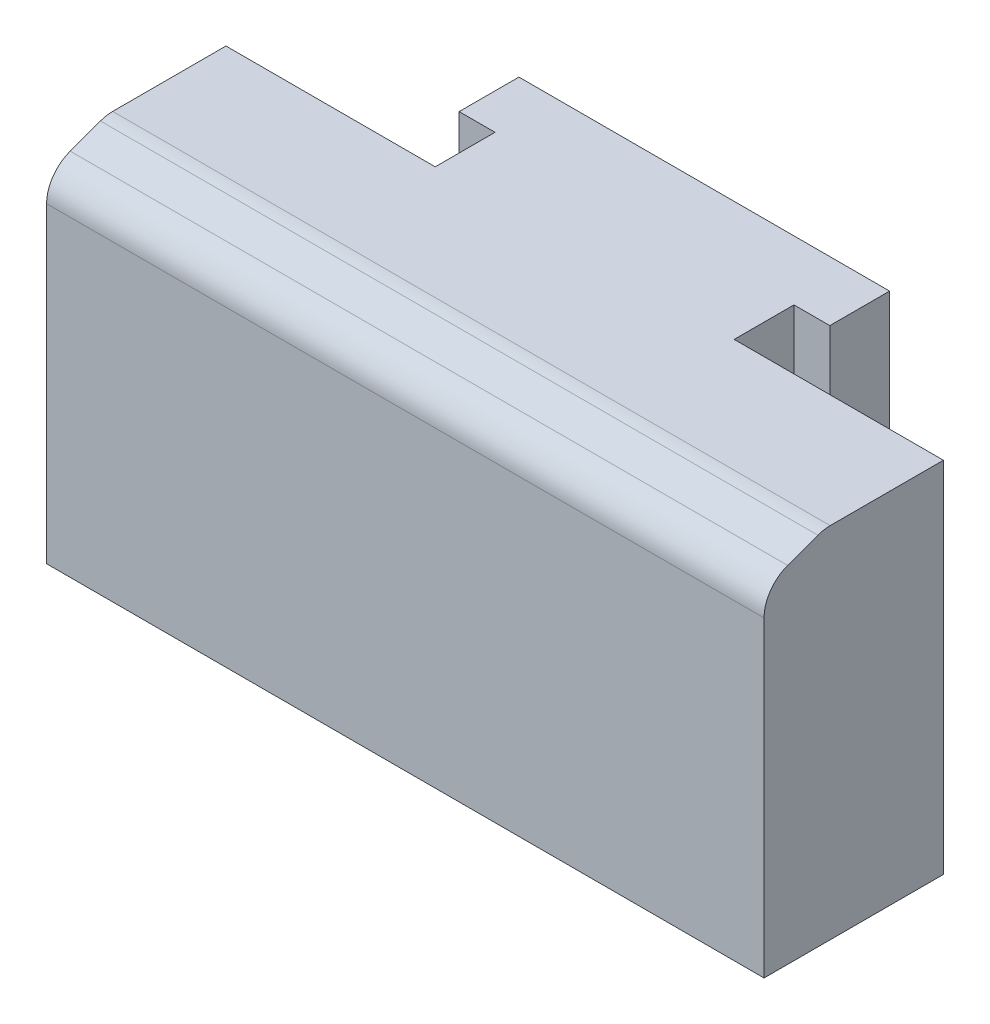
from build123d import *

# Parameters (mm, degrees)
SKETCH1_W              = 31
SKETCH1_H              = 30
BOSS_EXTRUDE1_DEPTH    = 25
SKETCH2_W              = 3
SKETCH2_H              = 20
CUT_EXTRUDE1_DEPTH     = 51.498103381
SKETCH3_W              = 17.5
SKETCH3_H              = 15
BOSS_EXTRUDE2_DEPTH    = 30
CHAMFER1_SIZE          = 5
CHAMFER1_SIZE2         = 1.819851171
FILLET1_R              = 3
M10_TAPPED_HOLE1_D     = 8.5
M10_TAPPED_HOLE1_DEPTH = 24.5
M10_TAPPED_HOLE1_TIP   = 2.553657631


with BuildPart() as part:
    # Sketch1 → Boss-Extrude1 (new body)
    with BuildSketch(Plane.XY):
        with Locations((-16.516533934, 15.197368421)):
            Rectangle(SKETCH1_W, SKETCH1_H)
    extrude(amount=BOSS_EXTRUDE1_DEPTH)

    # Sketch2 → Cut-Extrude1 (cut, through all)
    with BuildSketch(Plane.XZ.offset(-0.197368421)):
        with Locations((-30.516533934, 15)):
            Rectangle(SKETCH2_W, SKETCH2_H)
        with Locations((-2.516533934, 15)):
            Rectangle(SKETCH2_W, SKETCH2_H)
    extrude(amount=-CUT_EXTRUDE1_DEPTH, mode=Mode.SUBTRACT)

    # Sketch3 → Boss-Extrude2 (add, through all)
    with BuildSketch(Plane(origin=(0, 30.197368421, 0), x_dir=(1, 0, 0), z_dir=(0, 1, 0))):
        with Locations((4.733466066, -17.5)):
            Rectangle(SKETCH3_W, SKETCH3_H)
        with Locations((-37.766533934, -17.5)):
            Rectangle(SKETCH3_W, SKETCH3_H)
    extrude(amount=-BOSS_EXTRUDE2_DEPTH)

    # Chamfer1
    chamfer1_edges = [part.edges().sort_by_distance(p)[0] for p in [
        (-16.516533934, 30.197368421, 25),
    ]]
    chamfer1_side = [part.faces().sort_by_distance(p)[0] for p in [
        (-16.516533934, 30.197368421, 14.470338983),
    ]]
    chamfer(chamfer1_edges, length=CHAMFER1_SIZE, length2=CHAMFER1_SIZE2, reference=chamfer1_side[0])

    # Fillet1
    fillet1_edges = [part.edges().sort_by_distance(p)[0] for p in [
        (-16.516533934, 28.37751725, 25),
        (-16.516533934, 30.197368421, 20),
    ]]
    fillet(fillet1_edges, radius=FILLET1_R)

    # M10 Tapped Hole1
    with Locations(Plane(origin=(0, 0.197368421, 0), x_dir=(-1, 0, 0), z_dir=(0, -1, 0))):
        with Locations((16.516533934, -10)):
            Hole(M10_TAPPED_HOLE1_D / 2, depth=M10_TAPPED_HOLE1_DEPTH)
            with Locations((0, 0, -(M10_TAPPED_HOLE1_DEPTH + M10_TAPPED_HOLE1_TIP / 2))):  # 118° drill point
                Cone(0, M10_TAPPED_HOLE1_D / 2, M10_TAPPED_HOLE1_TIP, mode=Mode.SUBTRACT)


solid = part.part
